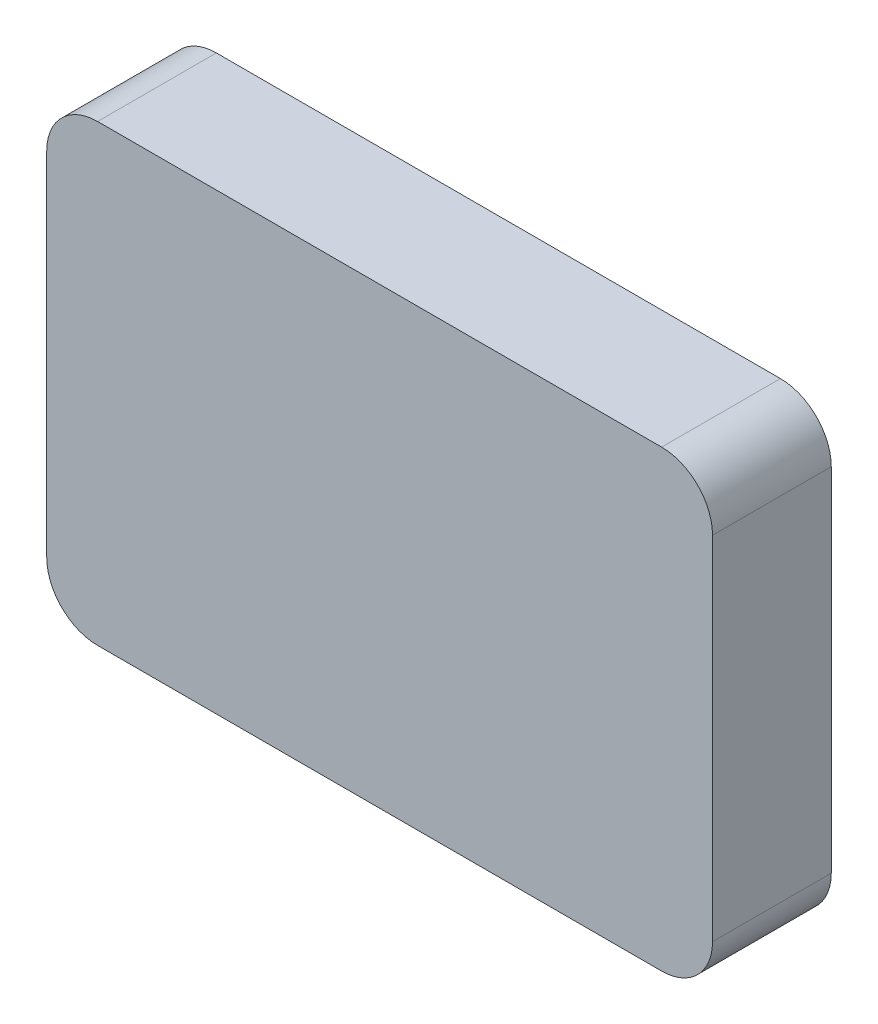
SolidWorks part; units mm, degrees
ref_plane "前视基准面" through (0, 0, 0) normal (0, 0, 1) x (1, 0, 0)
ref_plane "上视基准面" through (0, 0, 0) normal (0, 1, 0) x (1, 0, 0)
ref_plane "右视基准面" through (0, 0, 0) normal (1, 0, 0) x (0, 0, -1)
sketch "草图1" plane through (0, 0, 0) normal (0, 0, 1) x (1, 0, 0)
  line L1 (0, 0) -> (78.5, 0)
  line L2 (0, 0) -> (0, 53.5)
  line L3 (0, 53.5) -> (78.5, 53.5)
  line L4 (78.5, 0) -> (78.5, 53.5)
  dimension "D1" = 78.5
  dimension "D2" = 53.5
extrude "凸台-拉伸1" add sketch "草图1" along normal blind 14
fillet "圆角1" radius 6 4 edges at (78.5, 53.5, 7) (78.5, 0, 7) (0, 0, 7) (0, 53.5, 7)
